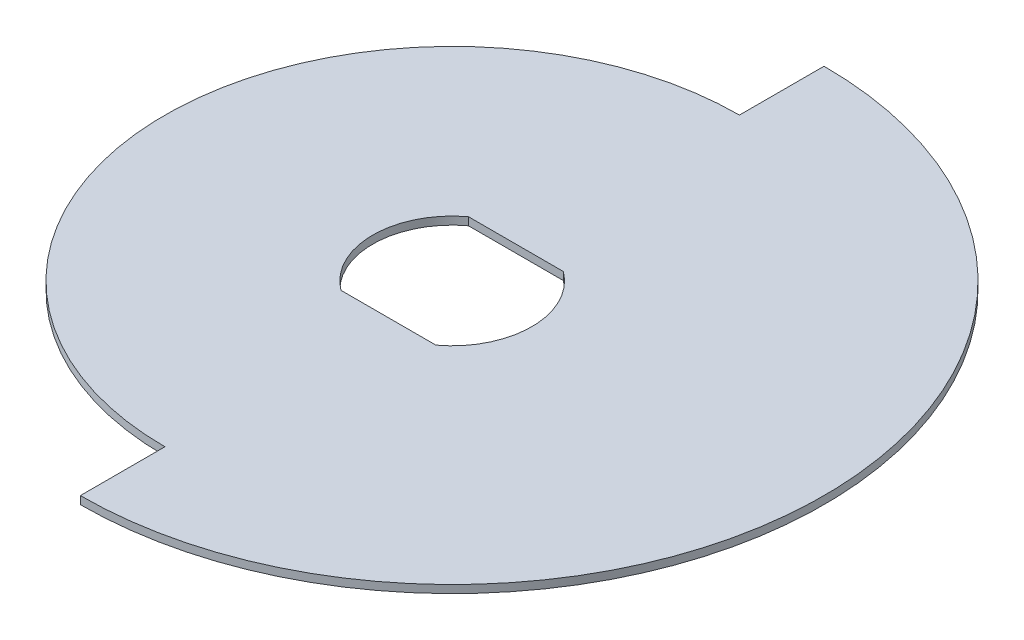
from build123d import *

# Parameters (mm, degrees)
SKETCH1_R           = 47.25
SKETCH1_R_2         = 10.1
BOSS_EXTRUDE1_DEPTH = 1
BOSS_EXTRUDE2_DEPTH = 1
CUT_EXTRUDE1_DEPTH  = 10


with BuildPart() as part:
    # Sketch1 → Boss-Extrude1 (new body)
    with BuildSketch(Plane(origin=(0, 0, 0), x_dir=(1, 0, 0), z_dir=(0, 1, 0))):
        with Locations(Location((0, 0, 0), (0, 0, 270))):
            Circle(SKETCH1_R)
        with Locations(Location((0, 0, 0), (0, 0, 270))):
            Circle(SKETCH1_R_2, mode=Mode.SUBTRACT)
    extrude(amount=BOSS_EXTRUDE1_DEPTH)

    # Sketch2 → Boss-Extrude2 (add)
    with BuildSketch(Plane.XZ):
        with BuildLine():
            Line((6.033241252, -8.1), (-6.033241252, -8.1))
            ThreePointArc((-6.033241252, -8.1), (0, -10.1), (6.033241252, -8.1))
        make_face()
        with BuildLine():
            Line((6.033241252, 8.1), (-6.033241252, 8.1))
            ThreePointArc((-6.033241252, 8.1), (0, 10.1), (6.033241252, 8.1))
        make_face()
    extrude(amount=-BOSS_EXTRUDE2_DEPTH)

    # Sketch3 → Cut-Extrude1 (cut)
    with BuildSketch(Plane.XZ):
        with BuildLine():
            Line((0, 47.25), (0, 36.5))
            ThreePointArc((0, 36.5), (-36.5, 0), (0, -36.5))
            Line((0, -36.5), (0, -47.25))
            ThreePointArc((0, -47.25), (-47.25, 0), (0, 47.25))
        make_face()
    extrude(amount=-CUT_EXTRUDE1_DEPTH, mode=Mode.SUBTRACT)


solid = part.part
